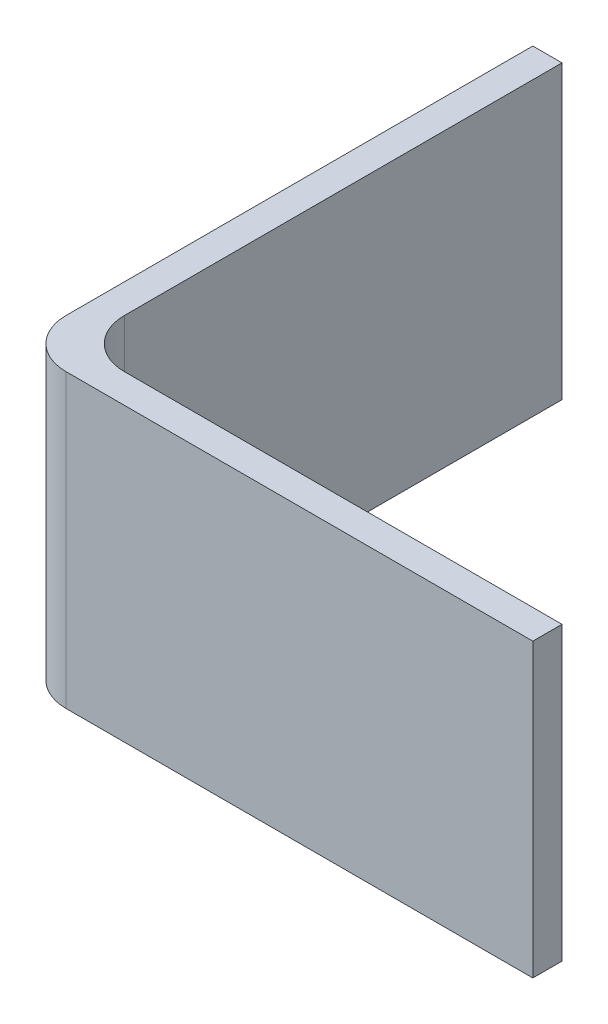
SolidWorks part; units mm, degrees
ref_plane "Front Plane" through (0, 0, 0) normal (0, 0, 1) x (1, 0, 0)
ref_plane "Top Plane" through (0, 0, 0) normal (0, 1, 0) x (1, 0, 0)
ref_plane "Right Plane" through (0, 0, 0) normal (1, 0, 0) x (0, 0, -1)
sketch "Sketch1" plane through (0, 0, 0) normal (0, 1, 0) x (1, 0, 0)
  line L0 (5, 0) -> (50, 0)
  line L1 (0, 5) -> (0, 50)
  line L2 (-3, 2) -> (-3, 50)
  line L3 (2, -3) -> (50, -3)
  line L4 (-3, 50) -> (0, 50)
  line L5 (50, 0) -> (50, -3)
  line L6 (0, 0) -> (50, 0) construction
  line L7 (0, 0) -> (0, 50) construction
  line L8 (-3, -3) -> (-3, 50) construction
  line L9 (-3, -3) -> (50, -3) construction
  arc A0 (5, 0) -> (0, 5) centre (5, 5) cw
  arc A1 (-3, 2) -> (2, -3) centre (2, 2) ccw
  point P10 (0, 0)
  dimension "D4" = 5
  dimension "D1" = 50
  dimension "D2" = 50
  dimension "D3" = 3
extrude "Boss-Extrude1" add sketch "Sketch1" along normal blind 30
